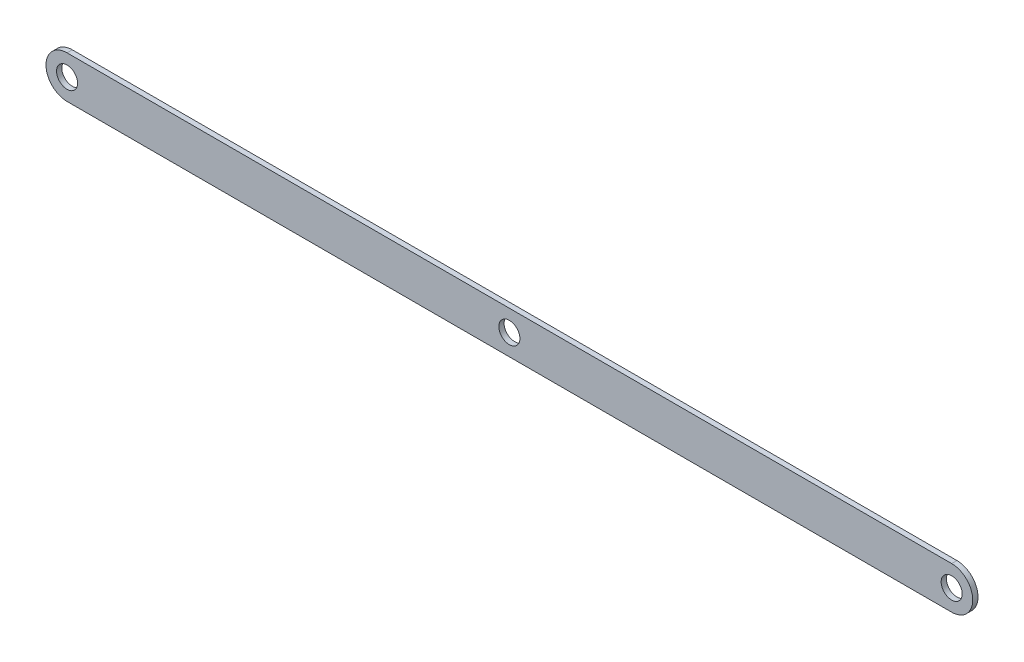
SolidWorks part; units mm, degrees
ref_plane "Front Plane" through (0, 0, 0) normal (0, 0, 1) x (1, 0, 0)
ref_plane "Top Plane" through (0, 0, 0) normal (0, 1, 0) x (1, 0, 0)
ref_plane "Right Plane" through (0, 0, 0) normal (1, 0, 0) x (0, 0, -1)
sketch "Sketch1" plane through (0, 0, 0) normal (0, 0, 1) x (1, 0, 0)
  line L0 (-210, 0) -> (210, 0) construction
  line L1 (-210, 10) -> (210, 10)
  line L2 (-210, -10) -> (210, -10)
  arc A0 (-210, 10) -> (-210, -10) centre (-210, 0) ccw
  arc A1 (210, -10) -> (210, 10) centre (210, 0) ccw
  circle A2 centre (-210, 0) radius 5
  circle A3 centre (210, 0) radius 5
  circle A4 centre (0, 0) radius 5
  point P2 (0, 0)
  dimension "D1" = 420
  dimension "D2" = 10
  dimension "D3" = 10
extrude "Boss-Extrude1" add sketch "Sketch1" along normal blind 2.5
